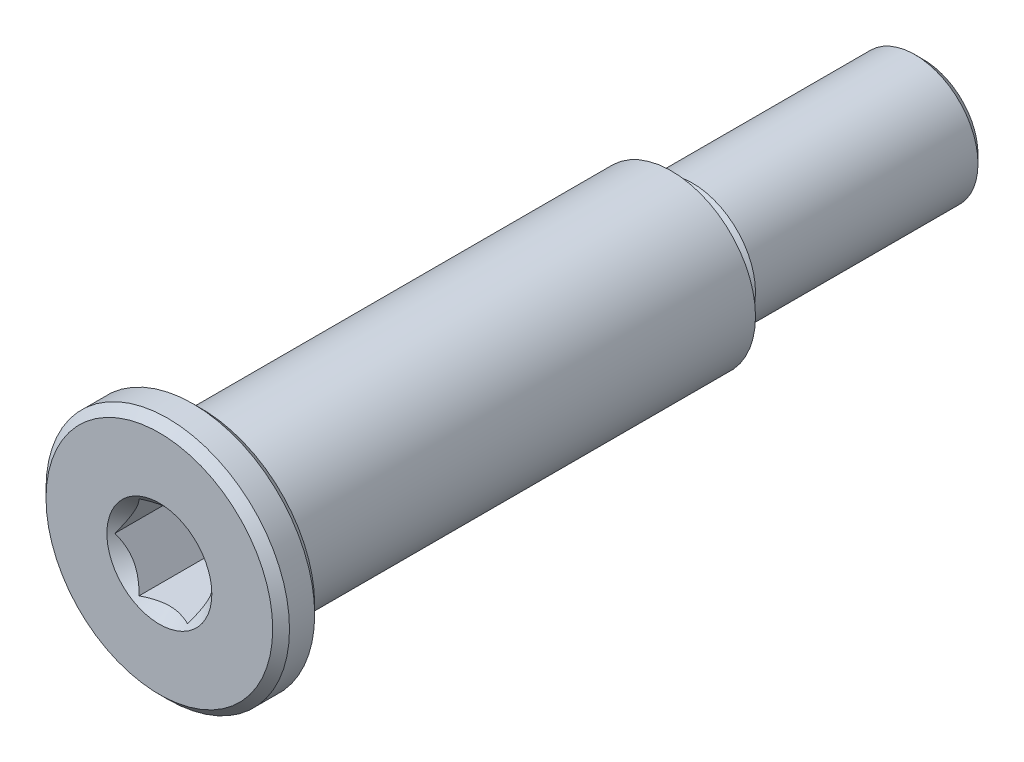
from build123d import *

# Parameters (mm, degrees)
SIZE_MM_DOWEL_HOLE1_D           = 2
SIZE_MM_DOWEL_HOLE1_DEPTH       = 2.5
SIZE_MM_DOWEL_HOLE1_CSINK_D     = 2.5
SIZE_MM_DOWEL_HOLE1_CSINK_ANGLE = 90
SIZE_MM_DOWEL_HOLE1_TIP         = 0.600860619
CUT_EXTRUDE1_DEPTH              = 2.5


with BuildPart() as part:
    # Sketch2 → Revolve1 (revolve)
    with BuildSketch(Plane(origin=(0, 0, 0), x_dir=(1, 0, 0), z_dir=(0, 1, 0))):
        Polygon((0, 0), (2.7, 0), (2.9, 0.2), (2.9, 0.8), (2.7, 1), (2, 1), (2, 12.2), (1.2, 12.2), (1.2, 12.4), (1.5, 12.7), (1.5, 18), (1.3, 18.2), (0, 18.2), align=None)
    revolve(axis=Axis((0, 0, 4.425925926), (0, 0, -1)))

    # Size mm Dowel Hole1
    with Locations(Plane.XY):
        with Locations((0, 0)):
            CounterSinkHole(SIZE_MM_DOWEL_HOLE1_D / 2, SIZE_MM_DOWEL_HOLE1_CSINK_D / 2, depth=SIZE_MM_DOWEL_HOLE1_DEPTH, counter_sink_angle=SIZE_MM_DOWEL_HOLE1_CSINK_ANGLE)
            with Locations((0, 0, -(SIZE_MM_DOWEL_HOLE1_DEPTH + SIZE_MM_DOWEL_HOLE1_TIP / 2))):  # 118° drill point
                Cone(0, SIZE_MM_DOWEL_HOLE1_D / 2, SIZE_MM_DOWEL_HOLE1_TIP, mode=Mode.SUBTRACT)

    # Sketch5 → Cut-Extrude1 (cut)
    with BuildSketch(Plane.XY):
        Polygon((0.577350269, -1), (1.154700538, 0), (0.577350269, 1), (-0.577350269, 1), (-1.154700538, 0), (-0.577350269, -1), align=None)
    extrude(amount=-CUT_EXTRUDE1_DEPTH, mode=Mode.SUBTRACT)


solid = part.part
